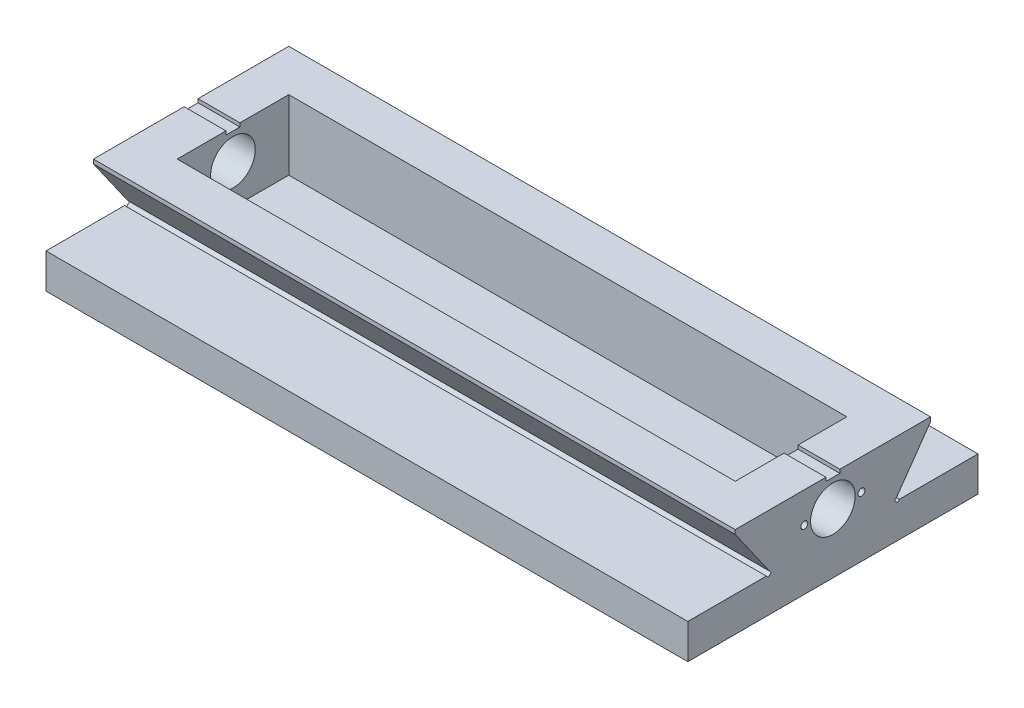
SolidWorks part; units mm, degrees
ref_plane "Front Plane" through (0, 0, 0) normal (0, 0, 1) x (1, 0, 0)
ref_plane "Top Plane" through (0, 0, 0) normal (0, 1, 0) x (1, 0, 0)
ref_plane "Right Plane" through (0, 0, 0) normal (1, 0, 0) x (0, 0, -1)
sketch "Sketch1" plane through (0, 0, 0) normal (1, 0, 0) x (0, 0, -1)
  line L0 (0, -12.5) -> (0, 73.8996) construction
  line L1 (-104, 12.5) -> (-47.7029, 12.5)
  line L2 (-104, 12.5) -> (-104, -12.5)
  line L3 (-104, -12.5) -> (104, -12.5)
  line L4 (104, 12.5) -> (104, -12.5)
  line L5 (-104, 12.5) -> (104, -12.5) construction
  line L6 (-104, -12.5) -> (104, 12.5) construction
  line L7 (-47.7029, 12.5) -> (-46.2977, 11.0769)
  line L8 (-46.2977, 11.0769) -> (-44.163, 13.1848)
  line L9 (-44.163, 13.1848) -> (-45.5683, 14.6079)
  line L10 (-45.5683, 14.6079) -> (-70, 49.5)
  line L11 (-70, 52.5) -> (-5, 52.5)
  line L12 (-5, 52.5) -> (-5, 49.9167)
  line L13 (-5, 49.9167) -> (5, 49.9167)
  line L14 (-70, 52.5) -> (-70, 49.5)
  line L15 (47.7029, 12.5) -> (104, 12.5)
  line L16 (70, 52.5) -> (70, 49.5)
  line L17 (5, 52.5) -> (5, 49.9167)
  line L18 (70, 52.5) -> (5, 52.5)
  line L19 (45.5683, 14.6079) -> (70, 49.5)
  line L20 (44.163, 13.1848) -> (45.5683, 14.6079)
  line L21 (46.2977, 11.0769) -> (44.163, 13.1848)
  line L22 (47.7029, 12.5) -> (46.2977, 11.0769)
  point P0 (0, 0)
  point P23 (0, 49.9167)
  dimension "D1" = 208
  dimension "D2" = 55
  dimension "D3" = 70
  dimension "D4" = 65
  dimension "D5" = 40
  dimension "D6" = 3
  dimension "D7" = 2
  dimension "D8" = 2
  dimension "D9" = 3
  dimension "D10" = 25
extrude "Boss-Extrude1" add sketch "Sketch1" along normal blind 460
sketch "Sketch2" plane through (0, 52.5, 0) normal (0, 1, 0) x (1, 0, 0)
  line L0 (0, 0) -> (460, 0) construction
  line L1 (460, 5) -> (460, -5) construction
  line L2 (230, 104) -> (230, -104) construction
  line L3 (460, 104) -> (0, 104) construction
  line L4 (460, -104) -> (0, -104) construction
  line L6 (30, 40) -> (430, 40)
  line L7 (30, 40) -> (30, -40)
  line L8 (30, -40) -> (430, -40)
  line L9 (430, 40) -> (430, -40)
  line L10 (30, 40) -> (430, -40) construction
  line L11 (30, -40) -> (430, 40) construction
  point P11 (230, 0)
  dimension "D1" = 80
  dimension "D2" = 400
extrude "Cut-Extrude1" cut sketch "Sketch2" against normal blind 50
sketch "Sketch3" plane through (460, 0, 0) normal (1, 0, 0) x (0, 0, -1)
  line L0 (0, 49.9167) -> (0, -12.5) construction
  line L1 (5, 49.9167) -> (-5, 49.9167) construction
  line L2 (-104, -12.5) -> (104, -12.5) construction
  line L3 (-5, 52.5) -> (-70, 52.5) construction
  circle A0 centre (0, 30.5) radius 16
  dimension "D1" = 32
  dimension "D2" = 22
extrude "Cut-Extrude2" cut sketch "Sketch3" against normal through all
hole_wizard "M6 Tapped Hole1" positions "Sketch4" profile "Sketch5" tap size "M6" standard "GB"
sketch "Sketch4" plane through (460, 0, 0) normal (1, 0, 0) x (0, 0, -1)
  point P0 (-20.5, 30.5)
  point P3 (20.5, 30.5)
sketch "Sketch5" plane through (460, 30.5, 20.5) normal (0, 1, 0) x (0, 0, -1)
  line L0 (0, 0) -> (0, 18.5022)
  line L1 (0, 18.5022) -> (2.5, 17)
  line L2 (2.5, 17) -> (2.5, 0)
  line L5 (2.5, 0) -> (0, 0)
  line L10 (0, 18.5022) -> (-2.5, 17) construction
  line L11 (0, -6.35) -> (0, 107.95) construction
  dimension "螺纹孔钻头直径" = 5
  dimension "螺纹孔钻头深度" = 17
  dimension "导头角度" = 118
cosmetic thread "Cosmetic Thread1" parameters "D1"=12, "D2"=6
cosmetic thread "Cosmetic Thread2" parameters "D1"=12, "D2"=6
hole_wizard "M6 Tapped Hole2" positions "Sketch6" profile "Sketch7" tap size "M6" standard "GB"
sketch "Sketch6" plane through (0, 0, 0) normal (-1, 0, 0) x (0, 0, 1)
  point P0 (17.4537, 19.7474)
  point P3 (-17.4537, 41.2526)
sketch "Sketch7" plane through (0, 19.7474, 17.4537) normal (0, 1, 0) x (0, 0, 1)
  line L0 (0, 0) -> (0, 18.5022)
  line L1 (0, 18.5022) -> (2.5, 17)
  line L2 (2.5, 17) -> (2.5, 0)
  line L5 (2.5, 0) -> (0, 0)
  line L10 (0, 18.5022) -> (-2.5, 17) construction
  line L11 (0, -6.35) -> (0, 107.95) construction
  dimension "螺纹孔钻头直径" = 5
  dimension "螺纹孔钻头深度" = 17
  dimension "导头角度" = 118
cosmetic thread "Cosmetic Thread3" parameters "D1"=12, "D2"=6
cosmetic thread "Cosmetic Thread4" parameters "D1"=12, "D2"=6
